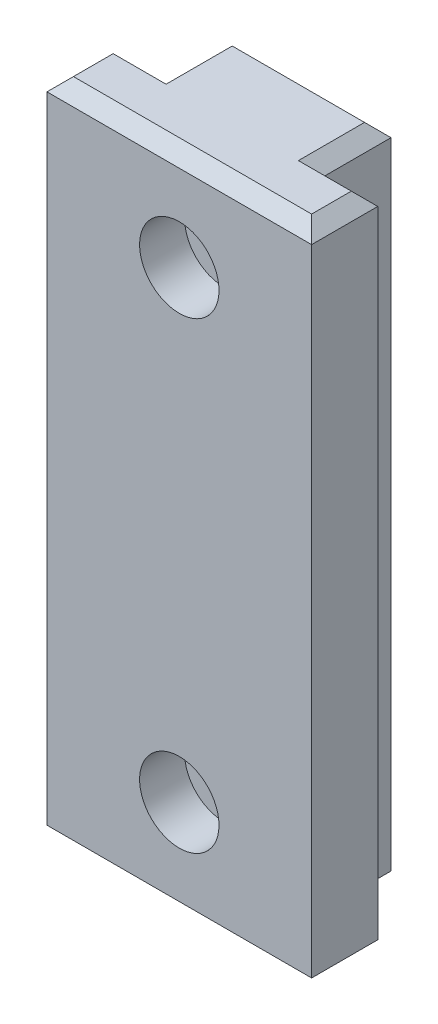
SolidWorks part; units mm, degrees
ref_plane "前视基准面" through (0, 0, 0) normal (0, 0, 1) x (1, 0, 0)
ref_plane "上视基准面" through (0, 0, 0) normal (0, 1, 0) x (1, 0, 0)
ref_plane "右视基准面" through (0, 0, 0) normal (1, 0, 0) x (0, 0, -1)
sketch "草图1" plane through (0, 0, 0) normal (0, 1, 0) x (1, 0, 0)
  line L0 (10, 0) -> (-10, 0)
  line L1 (-10, 0) -> (-10, 5)
  line L2 (-10, 5) -> (-6, 5)
  line L3 (-6, 5) -> (-6, 10)
  line L4 (-6, 10) -> (6, 10)
  line L5 (0, 0) -> (0, 11.8054) construction
  line L6 (6, 5) -> (6, 10)
  line L7 (10, 5) -> (6, 5)
  line L8 (10, 0) -> (10, 5)
  point P8 (0, 10)
  dimension "D1" = 12
  dimension "D2" = 20
  dimension "D3" = 10
  dimension "D4" = 5
extrude "凸台-拉伸1" add sketch "草图1" along normal blind 50
chamfer "倒角1" distance 1 angle 45 16 edges at (0, 50, 0) (-10, 50, -2.5) (-8, 50, -5) (-6, 50, -7.5) (0, 50, -10) (6, 50, -7.5) (8, 50, -5) (10, 50, -2.5) (-10, 0, -2.5) (-8, 0, -5) (-6, 0, -7.5) (10, 0, -2.5) (8, 0, -5) (6, 0, -7.5) (0, 0, -10) (0, 0, 0)
sketch "草图4" plane through (0, 0, 0) normal (0, 0, 1) x (1, 0, 0)
  line L0 (0, 0) -> (0, 50) construction
  line L1 (-9, 50) -> (9, 50) construction
  point P0 (0, 42.5)
  point P2 (0, 7.5)
  dimension "D1" = 7.5
  dimension "D2" = 35
hole_wizard "M3 六角圆柱头螺钉的柱形沉头孔1" positions "草图4" profile "草图3" counterbore size "M3" standard "GB" end condition through all
sketch "草图3" plane through (0, 42.5, 0) normal (1, 0, 0) x (0, -1, 0)
  line L0 (0, 0) -> (0, 10)
  line L1 (0, 10) -> (1.7, 10)
  line L3 (1.7, 10) -> (1.7, 3.4)
  line L4 (1.7, 3.4) -> (3, 3.4)
  line L5 (3, 3.4) -> (3, 0)
  line L7 (3, 0) -> (0, 0)
  line L11 (0, -6.35) -> (0, 107.95) construction
  dimension "通孔孔直径" = 3.4
  dimension "通孔孔深度" = 10
  dimension "柱形沉头孔直径" = 6
  dimension "柱形沉头孔深度" = 3.4
